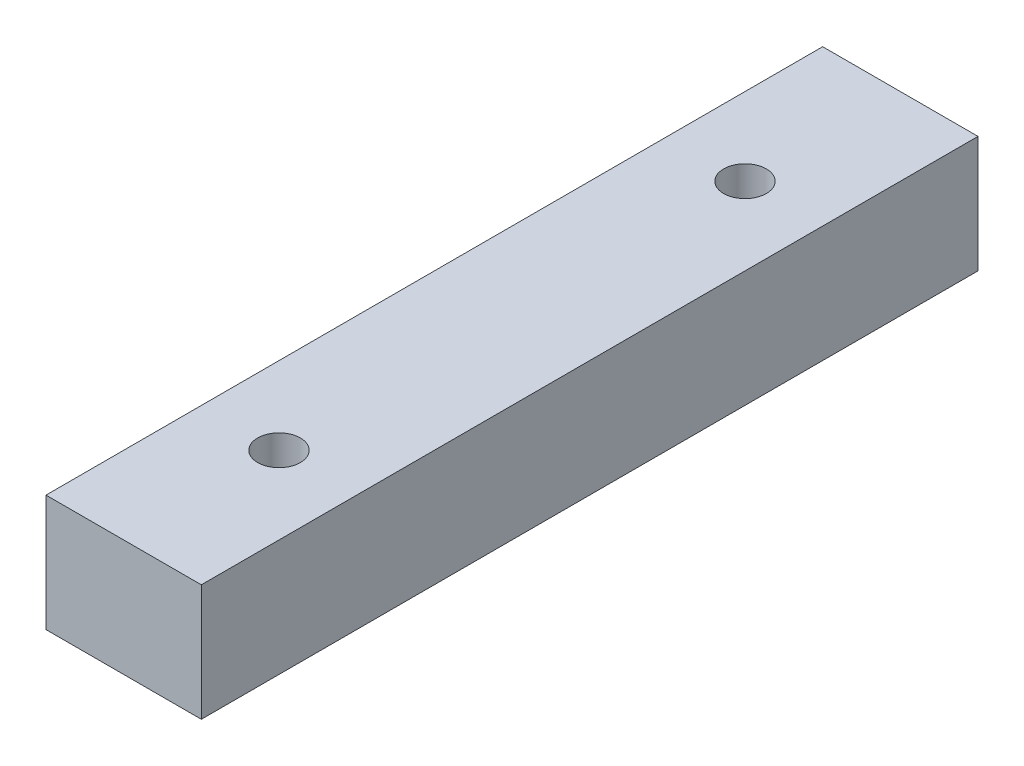
SolidWorks part; units mm, degrees
material "PU "
ref_plane "前基準面" through (0, 0, 0) normal (0, 0, 1) x (1, 0, 0)
ref_plane "上基準面" through (0, 0, 0) normal (0, 1, 0) x (1, 0, 0)
ref_plane "右基準面" through (0, 0, 0) normal (1, 0, 0) x (0, 0, -1)
sketch "草图1" plane through (0, 0, 0) normal (0, 1, 0) x (1, 0, 0)
  line L1 (-20, -100) -> (20, -100)
  line L2 (-20, -100) -> (-20, 100)
  line L3 (-20, 100) -> (20, 100)
  line L4 (20, -100) -> (20, 100)
  line L5 (-20, -100) -> (20, 100) construction
  line L6 (-20, 100) -> (20, -100) construction
  point P0 (0, 0)
  dimension "D1" = 40
  dimension "D2" = 200
extrude "凸台-拉伸1" add sketch "草图1" along normal mid plane 30
hole_wizard "打孔尺寸(%根据)内六角圆柱头螺钉的类型1" positions "草图2" profile "草图3" counterbore size "M6" standard "GB" end condition through all
sketch "草图2" plane through (0, 15, 0) normal (0, 1, 0) x (1, 0, 0)
  line L0 (0, 0) -> (34.6227, 0) construction
  point P0 (0, 60)
  point P8 (0, -60)
  dimension "D1" = 120
sketch "草图3" plane through (0, 15, -60) normal (1, 0, 0) x (0, 0, 1)
  line L0 (0, 0) -> (0, 30)
  line L1 (0, 30) -> (3.3, 30)
  line L3 (3.3, 30) -> (3.3, 10)
  line L4 (3.3, 10) -> (5.5, 10)
  line L5 (5.5, 10) -> (5.5, 0)
  line L7 (5.5, 0) -> (0, 0)
  line L11 (0, -6.35) -> (0, 107.95) construction
  dimension "通孔孔直径" = 6.6
  dimension "通孔孔深度" = 30
  dimension "柱形沉头孔直径" = 11
  dimension "柱形沉头孔深度" = 10
